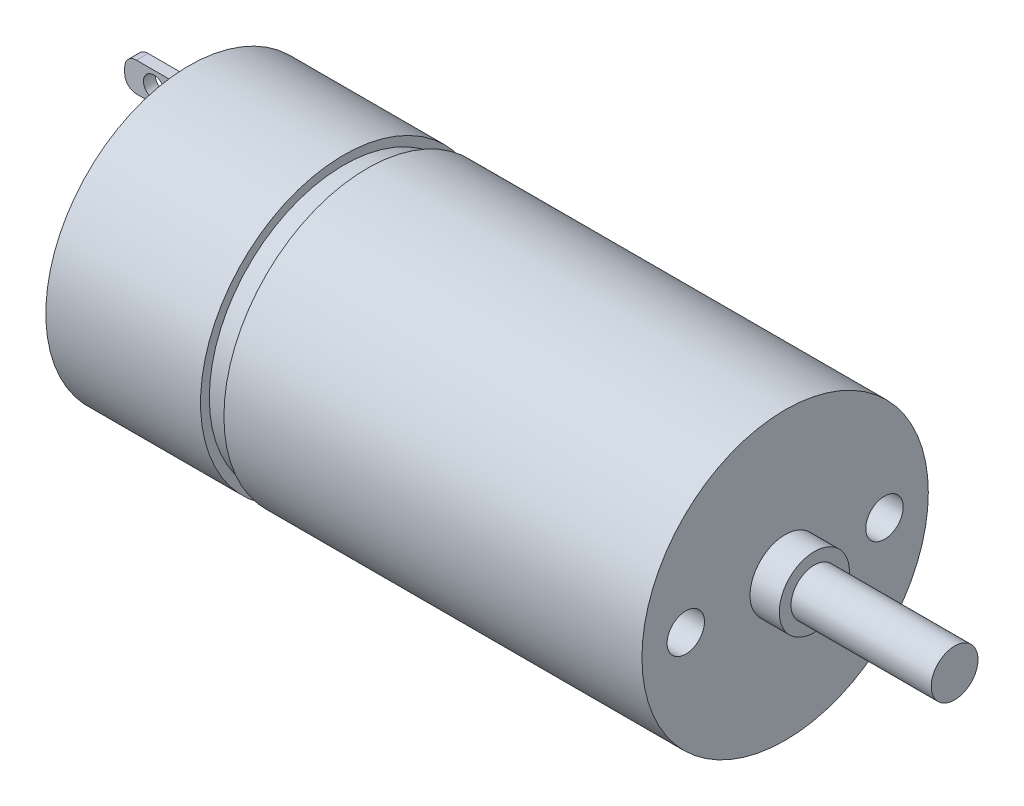
from build123d import *

# Parameters (mm, degrees)
SKETCH4_R           = 12.25
BOSS_EXTRUDE1_DEPTH = 51
SKETCH5_W           = 5
SKETCH5_H           = 2.5
SKETCH5_R           = 0.9
BOSS_EXTRUDE2_DEPTH = 0.5
FILLET1_R           = 1
SKETCH6_R           = 3
BOSS_EXTRUDE3_DEPTH = 2.5
SKETCH7_R           = 2
BOSS_EXTRUDE4_DEPTH = 12
SKETCH8_W           = 2
SKETCH8_H           = 3.5
SKETCH9_R           = 1.6
CUT_EXTRUDE1_DEPTH  = 5


with BuildPart() as part:
    # Sketch4 → Boss-Extrude1 (new body)
    with BuildSketch(Plane(origin=(0, 0, 0), x_dir=(0, 0, -1), z_dir=(1, 0, 0))):
        Circle(SKETCH4_R)
    extrude(amount=BOSS_EXTRUDE1_DEPTH)

    # Sketch5 → Boss-Extrude2 (add, symmetric)
    # profile 1 of 2: a face of its own
    with BuildSketch(Plane.XY):
        with Locations((-2.5, 9.653593257)):
            Rectangle(SKETCH5_W, SKETCH5_H)
        with Locations((-2.5, 9.653593257)):
            Circle(SKETCH5_R, mode=Mode.SUBTRACT)
    # profile 2 of 2: a face of its own
    with BuildSketch(Plane.XY):
        with Locations((-2.5, -9.653593257)):
            Rectangle(SKETCH5_W, SKETCH5_H)
        with Locations(Location((-2.5, -9.653593257, 0), (0, 0, 180))):
            Circle(SKETCH5_R, mode=Mode.SUBTRACT)
    extrude(amount=BOSS_EXTRUDE2_DEPTH, both=True)

    # Fillet1
    fillet1_edges = [part.edges().sort_by_distance(p)[0] for p in [
        (-5, 8.403593257, 0),
        (-5, -8.403593257, 0),
        (-5, -10.903593257, 0),
        (-5, 10.903593257, 0),
    ]]
    fillet(fillet1_edges, radius=FILLET1_R)

    # Sketch6 → Boss-Extrude3 (add)
    with BuildSketch(Plane(origin=(51, 0, 0), x_dir=(0, 0, -1), z_dir=(1, 0, 0))):
        Circle(SKETCH6_R)
    extrude(amount=BOSS_EXTRUDE3_DEPTH)

    # Sketch7 → Boss-Extrude4 (add)
    with BuildSketch(Plane(origin=(53.5, 0, 0), x_dir=(0, 0, -1), z_dir=(1, 0, 0))):
        Circle(SKETCH7_R)
    extrude(amount=BOSS_EXTRUDE4_DEPTH)

    # Sketch8 → Cut-Revolve1 (revolve, cut)
    with BuildSketch(Plane.XY, mode=Mode.PRIVATE) as cut_revolve1_sk:
        with Locations((14.235706655, 13.25)):
            Rectangle(SKETCH8_W, SKETCH8_H)
    revolve(cut_revolve1_sk.sketch.rotate(Axis((-4.366287434, 0, 0), (1, 0, 0)), 90), axis=Axis((-4.366287434, 0, 0), (1, 0, 0)), mode=Mode.SUBTRACT)

    # Sketch9 → Cut-Extrude1 (cut)
    with BuildSketch(Plane(origin=(51, 0, 0), x_dir=(0, 0, -1), z_dir=(1, 0, 0))):
        with Locations((-8.5, 0)):
            Circle(SKETCH9_R)
        with Locations((8.5, 0)):
            Circle(SKETCH9_R)
    extrude(amount=-CUT_EXTRUDE1_DEPTH, mode=Mode.SUBTRACT)


solid = part.part
